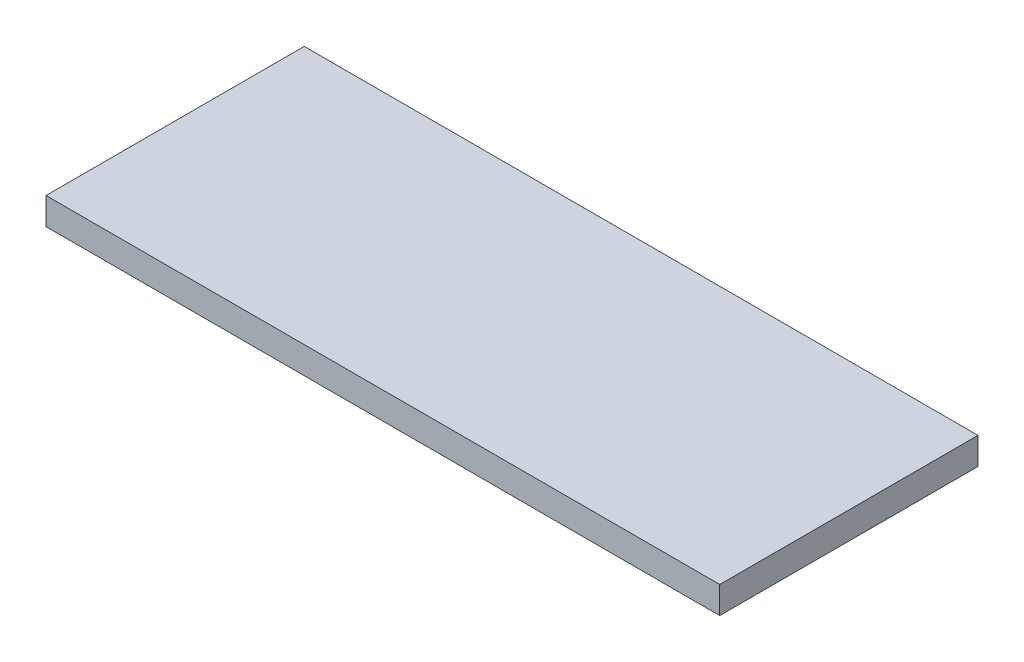
from build123d import *

# Parameters (mm, degrees)
SKETCH_1_W      = 300
SKETCH_1_H      = 115
EXTRUDE_1_DEPTH = 12


with BuildPart() as part:
    # 草图1 → 凸台-拉伸1 (new body)
    with BuildSketch(Plane(origin=(0, 0, 0), x_dir=(1, 0, 0), z_dir=(0, 1, 0))):
        Rectangle(SKETCH_1_W, SKETCH_1_H)
    extrude(amount=EXTRUDE_1_DEPTH)


solid = part.part
